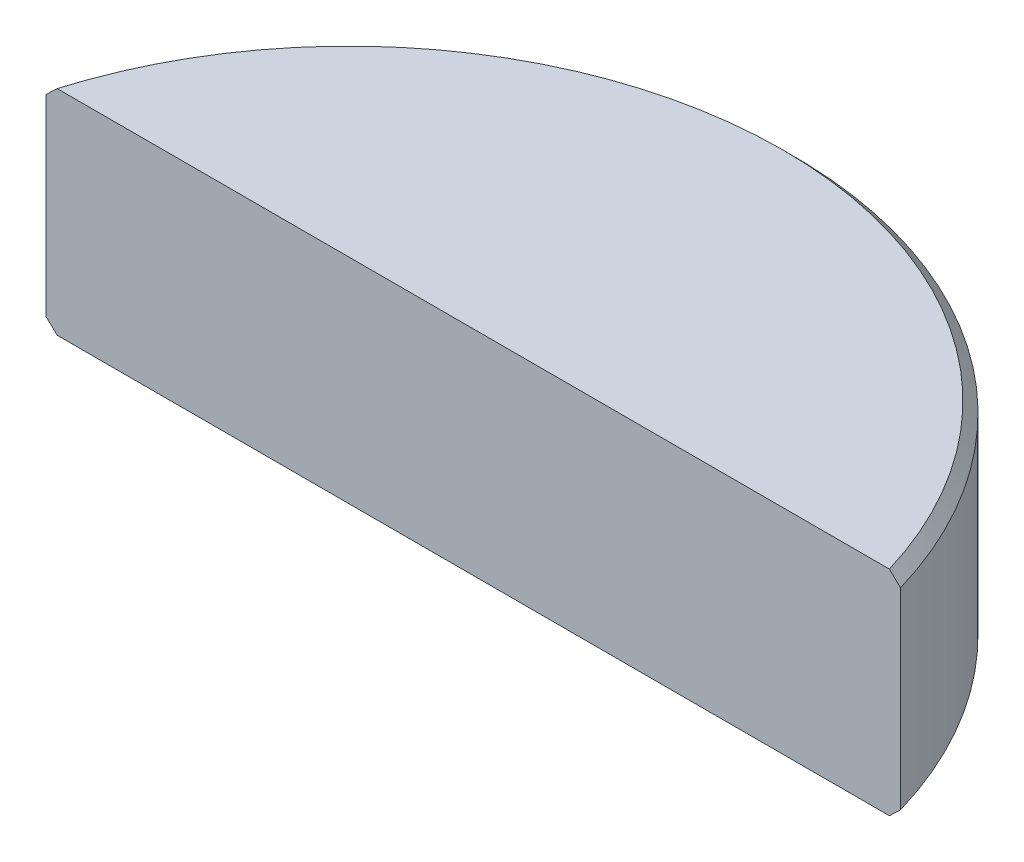
SolidWorks part; units mm, degrees
ref_plane "Front Plane" through (0, 0, 0) normal (0, 0, 1) x (1, 0, 0)
ref_plane "Top Plane" through (0, 0, 0) normal (0, 1, 0) x (1, 0, 0)
ref_plane "Right Plane" through (0, 0, 0) normal (1, 0, 0) x (0, 0, -1)
other "Configuration Table"
ref_plane "Plane1" through (0, -3, 0) normal (0, -1, 0) x (1, 0, 0)
sketch "Sketch1" plane through (0, -3, 0) normal (0, -1, 0) x (1, 0, 0)
  line L0 (12, 0) -> (-12, 0)
  arc A0 (-12, 0) -> (12, 0) centre (0, 3.5) ccw
  dimension "D1" = 12.5
  dimension "D2" = 12
extrude "Boss-Extrude1" add sketch "Sketch1" against normal blind 6
chamfer "Chamfer1" distance 0.3 angle 45 2 edges at (0, -3, -9) (0, 3, -9)
